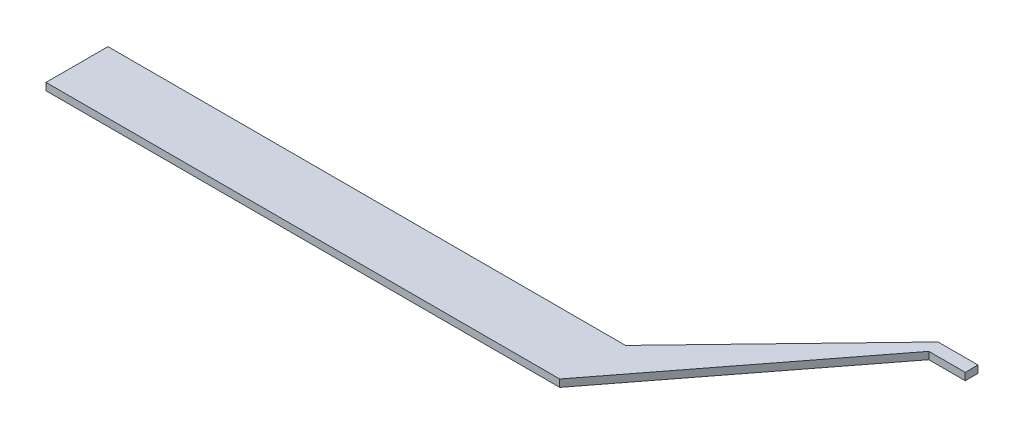
from build123d import *

# Parameters (mm, degrees)
BOSS_EXTRUDE1_DEPTH = 0.2


with BuildPart() as part:
    # Sketch1 → Boss-Extrude1 (new body)
    with BuildSketch(Plane(origin=(0, 0, 0), x_dir=(1, 0, 0), z_dir=(0, 1, 0))):
        Polygon((14.2, 1.7), (18.405344965, 6.07), (19.5, 6.07), (19.5, 5.72), (18.5, 5.72), (14.095006994, 0), (0, 0), (0, 1.7), align=None)
    extrude(amount=BOSS_EXTRUDE1_DEPTH)


solid = part.part
